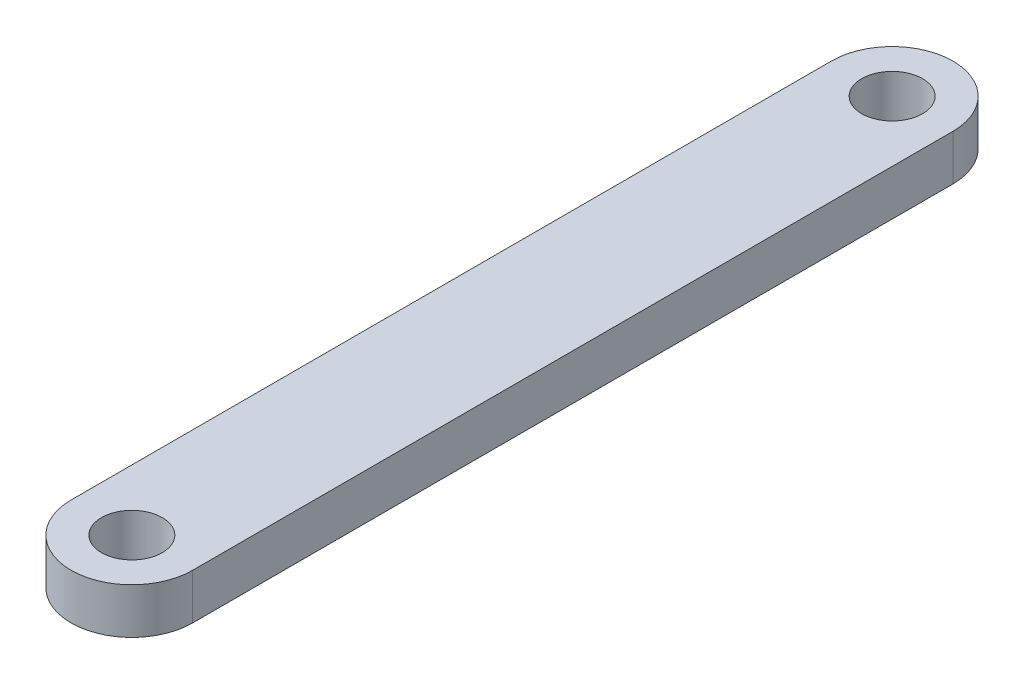
SolidWorks part; units mm, degrees
ref_plane "Front" through (0, 0, 0) normal (0, 0, 1) x (1, 0, 0)
ref_plane "Top" through (0, 0, 0) normal (0, 1, 0) x (1, 0, 0)
ref_plane "Right" through (0, 0, 0) normal (1, 0, 0) x (0, 0, -1)
sketch "Sketch1" plane through (0, 0, 0) normal (0, 1, 0) x (1, 0, 0)
  line L0 (0, 0) -> (0, 250) construction
  line L1 (-20, 0) -> (-20, 250)
  line L2 (20, 0) -> (20, 250)
  arc A0 (-20, 0) -> (20, 0) centre (0, 0) ccw
  arc A1 (20, 250) -> (-20, 250) centre (0, 250) ccw
  circle A2 centre (0, 250) radius 10
  circle A3 centre (0, 0) radius 10
  point P3 (0, 125)
  dimension "D2" = 20
  dimension "D3" = 20
  dimension "D4" = 20
  dimension "D1" = 250
extrude "Boss-Extrude1" add sketch "Sketch1" along normal blind 15
